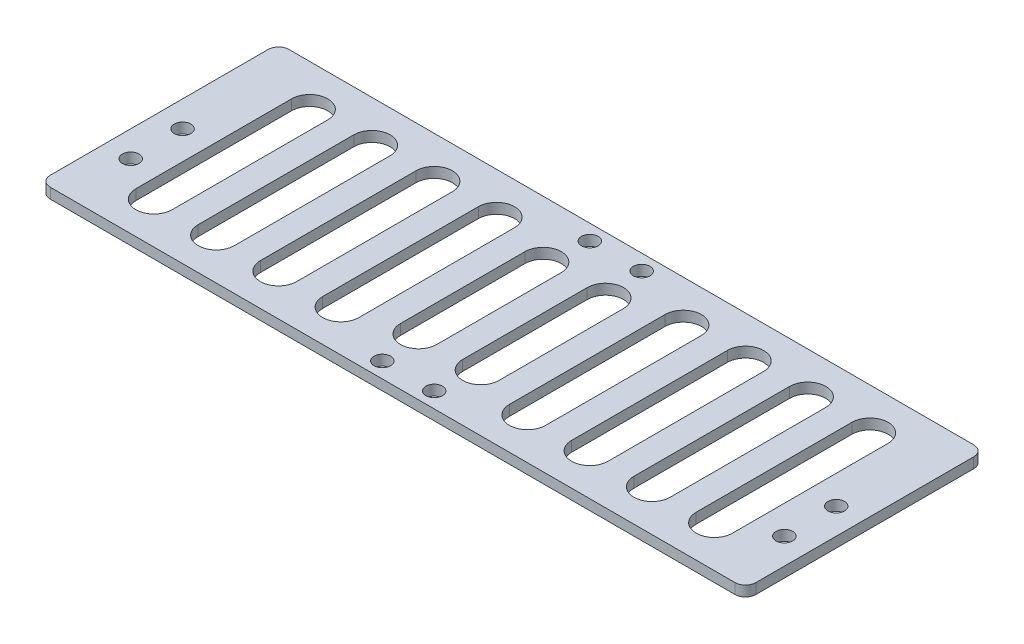
SolidWorks part; units mm, degrees
material "Thornel Mat VMA"
ref_plane "前视基准面" through (0, 0, 0) normal (0, 0, 1) x (1, 0, 0)
ref_plane "上视基准面" through (0, 0, 0) normal (0, 1, 0) x (1, 0, 0)
ref_plane "右视基准面" through (0, 0, 0) normal (1, 0, 0) x (0, 0, -1)
sketch "草图1" plane through (0, 0, 0) normal (0, 1, 0) x (1, 0, 0)
  line L0 (0, 23) -> (0, -23) construction
  line L1 (68, -23) -> (-68, -23)
  line L2 (68, -23) -> (68, 23)
  line L3 (68, 23) -> (-68, 23)
  line L4 (-68, -23) -> (-68, 23)
  line L5 (68, -23) -> (-68, 23) construction
  line L6 (68, 23) -> (-68, -23) construction
  line L7 (-63, -0.5) -> (-63, -10.5) construction
  line L8 (-5, -20) -> (5, -20) construction
  line L10 (63, -0.5) -> (63, -10.5) construction
  line L11 (-68, 0) -> (68, 0) construction
  line L13 (-5, 20) -> (5, 20) construction
  circle A0 centre (-63, -0.5) radius 1.6
  circle A1 centre (-63, -10.5) radius 1.6
  circle A2 centre (-5, -20) radius 1.6
  circle A3 centre (5, -20) radius 1.6
  circle A6 centre (63, -10.5) radius 1.6
  circle A7 centre (63, -0.5) radius 1.6
  circle A10 centre (5, 20) radius 1.6
  circle A11 centre (-5, 20) radius 1.6
  point P0 (0, 0)
  dimension "D2" = 12.5
  dimension "D4" = 3.2
  dimension "D1" = 136
  dimension "D3" = 10
  dimension "D5" = 5
  dimension "D6" = 3
  dimension "D7" = 46
extrude "凸台-拉伸1" add sketch "草图1" along normal blind 2
sketch "草图2" plane through (0, 2, 0) normal (0, 1, 0) x (1, 0, 0)
  line L0 (0, 23) -> (0, -23) construction
  line L1 (68, 23) -> (-68, 23) construction
  line L2 (-68, -23) -> (68, -23) construction
  line L3 (-68, 0) -> (68, 0) construction
  line L4 (-68, 23) -> (-68, -23) construction
  line L5 (68, -23) -> (68, 23) construction
  line L6 (-54, 15) -> (-54, -15) construction
  line L7 (-50.5, 15) -> (-50.5, -15)
  line L8 (-57.5, 15) -> (-57.5, -15)
  line L9 (-42, 15) -> (-42, -15) construction
  line L10 (-38.5, 15) -> (-38.5, -15)
  line L11 (-45.5, 15) -> (-45.5, -15)
  line L12 (-30, 15) -> (-30, -15) construction
  line L13 (-26.5, 15) -> (-26.5, -15)
  line L14 (-33.5, 15) -> (-33.5, -15)
  line L15 (-18, 15) -> (-18, -15) construction
  line L16 (-14.5, 15) -> (-14.5, -15)
  line L17 (-21.5, 15) -> (-21.5, -15)
  line L18 (-6, 12) -> (-6, -12) construction
  line L19 (-2.5, 12) -> (-2.5, -12)
  line L20 (-9.5, 12) -> (-9.5, -12)
  line L21 (6, 12) -> (6, -12) construction
  line L22 (9.5, 12) -> (9.5, -12)
  line L23 (2.5, 12) -> (2.5, -12)
  line L24 (18, 15) -> (18, -15) construction
  line L25 (21.5, 15) -> (21.5, -15)
  line L26 (14.5, 15) -> (14.5, -15)
  line L27 (30, 15) -> (30, -15) construction
  line L28 (33.5, 15) -> (33.5, -15)
  line L29 (26.5, 15) -> (26.5, -15)
  line L30 (42, 15) -> (42, -15) construction
  line L31 (45.5, 15) -> (45.5, -15)
  line L32 (38.5, 15) -> (38.5, -15)
  line L33 (54, 15) -> (54, -15) construction
  line L34 (57.5, 15) -> (57.5, -15)
  line L35 (50.5, 15) -> (50.5, -15)
  arc A0 (-50.5, 15) -> (-57.5, 15) centre (-54, 15) ccw
  arc A1 (-57.5, -15) -> (-50.5, -15) centre (-54, -15) ccw
  arc A2 (-38.5, 15) -> (-45.5, 15) centre (-42, 15) ccw
  arc A3 (-45.5, -15) -> (-38.5, -15) centre (-42, -15) ccw
  arc A4 (-26.5, 15) -> (-33.5, 15) centre (-30, 15) ccw
  arc A5 (-33.5, -15) -> (-26.5, -15) centre (-30, -15) ccw
  arc A6 (-14.5, 15) -> (-21.5, 15) centre (-18, 15) ccw
  arc A7 (-21.5, -15) -> (-14.5, -15) centre (-18, -15) ccw
  arc A8 (-2.5, 12) -> (-9.5, 12) centre (-6, 12) ccw
  arc A9 (-9.5, -12) -> (-2.5, -12) centre (-6, -12) ccw
  arc A10 (9.5, 12) -> (2.5, 12) centre (6, 12) ccw
  arc A11 (2.5, -12) -> (9.5, -12) centre (6, -12) ccw
  arc A12 (21.5, 15) -> (14.5, 15) centre (18, 15) ccw
  arc A13 (14.5, -15) -> (21.5, -15) centre (18, -15) ccw
  arc A14 (33.5, 15) -> (26.5, 15) centre (30, 15) ccw
  arc A15 (26.5, -15) -> (33.5, -15) centre (30, -15) ccw
  arc A16 (45.5, 15) -> (38.5, 15) centre (42, 15) ccw
  arc A17 (38.5, -15) -> (45.5, -15) centre (42, -15) ccw
  arc A18 (57.5, 15) -> (50.5, 15) centre (54, 15) ccw
  arc A19 (50.5, -15) -> (57.5, -15) centre (54, -15) ccw
  point P14 (-54, 0)
  point P22 (-42, 0)
  point P29 (-30, 0)
  point P36 (-18, 0)
  point P43 (-6, 0)
  point P50 (6, 0)
  point P57 (18, 0)
  point P64 (30, 0)
  point P71 (42, 0)
  point P78 (54, 0)
  dimension "D1" = 3.5
  dimension "D2" = 30
  dimension "D4" = 12
  dimension "D3" = 24
extrude "切除-拉伸1" cut sketch "草图2" against normal through all
fillet "R2 圆角1" radius 2 4 edges at (-68, 1, 23) (68, 1, 23) (68, 1, -23) (-68, 1, -23)
